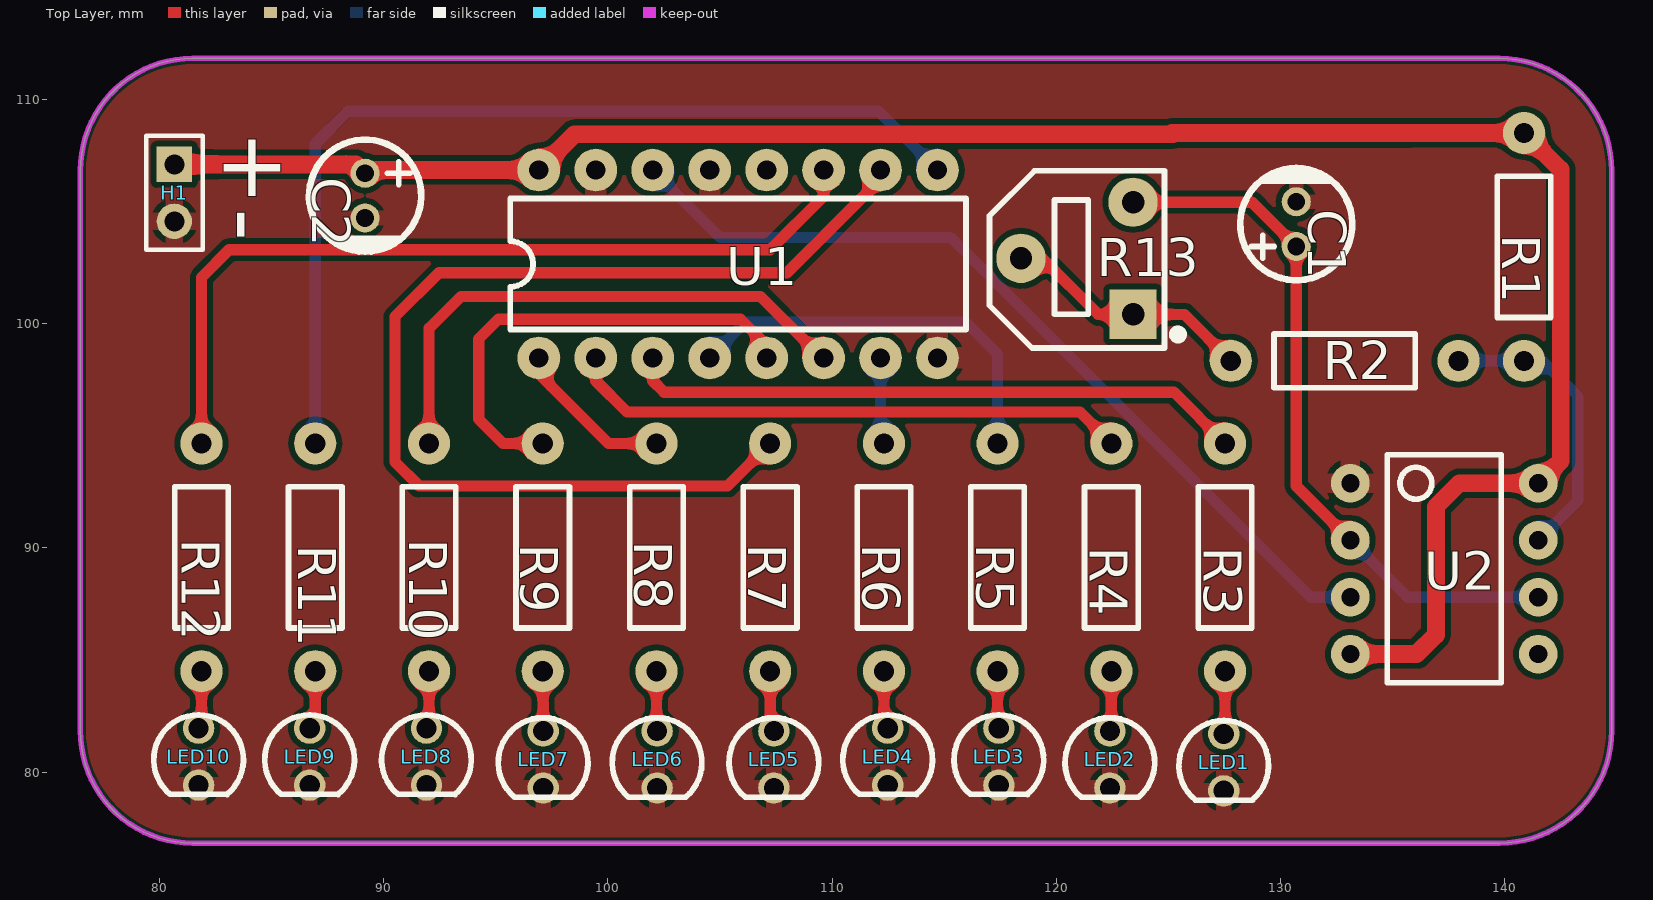
[diagram p0: Top Layer view]
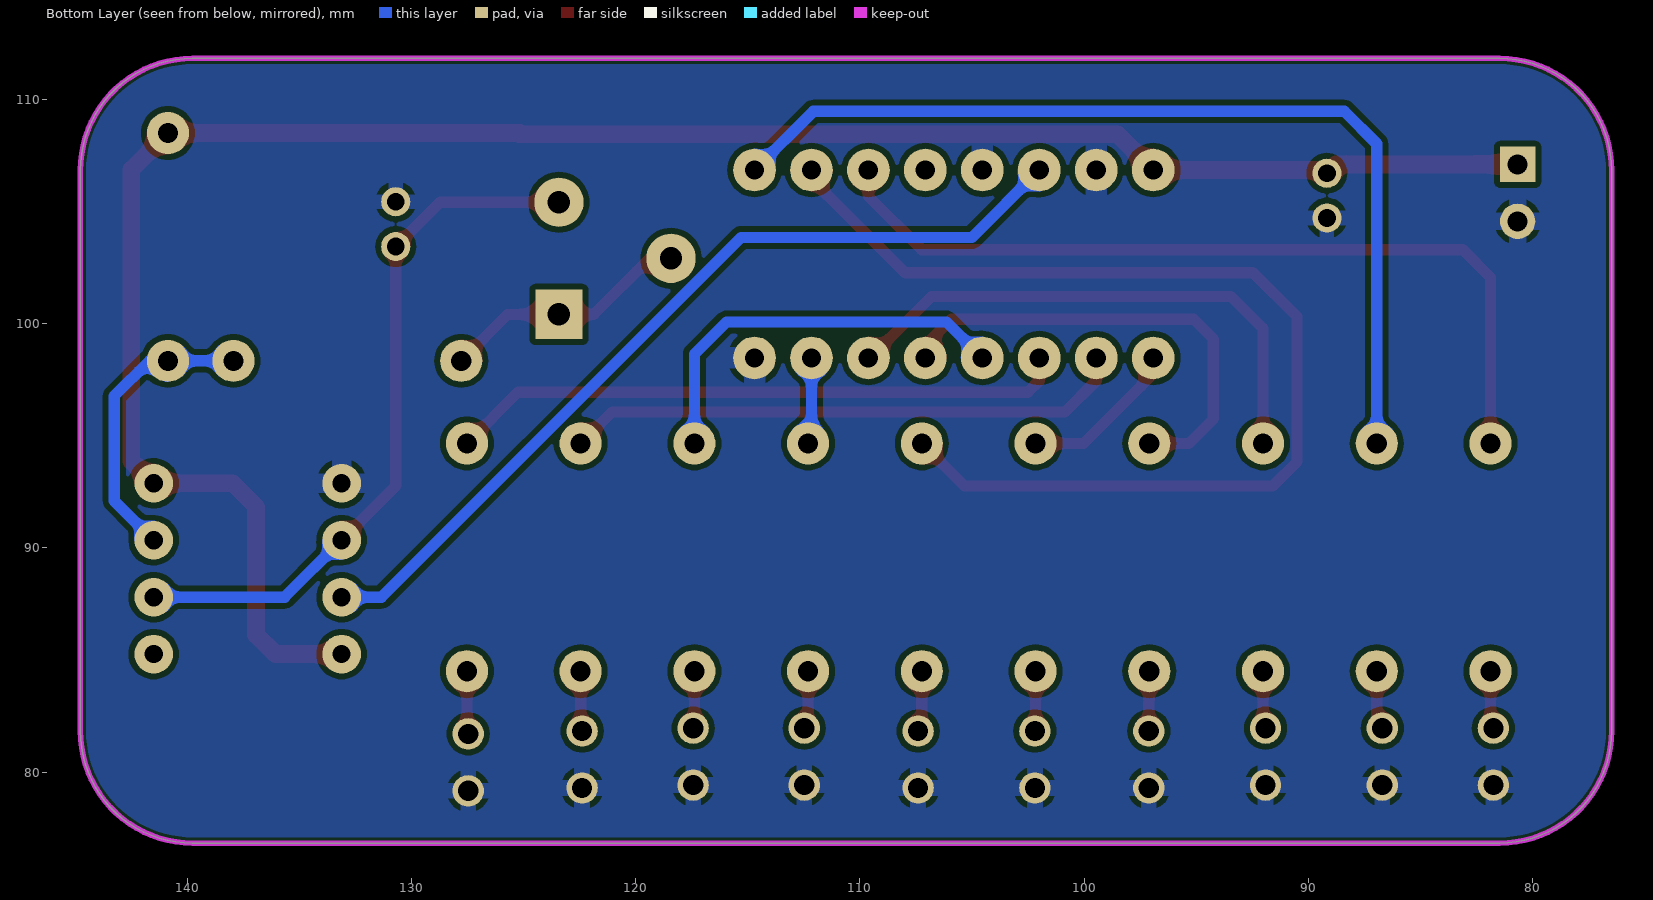
[diagram p1: Bottom Layer view, seen from below]
# Altium PCB MISC49871.pcbdoc
Units mm, origin at the board's own origin, x right, y up, seen from the top; angles counter-clockwise.
Board outline 68.29 x 35 mm, 2 copper layers (Top Layer, Bottom Layer), stack 1.58 mm thick; 28 components, 26 nets, 77 pads, 0 vias.

## Layer stack, top to bottom
Top Solder Mask Layer: solder mask 0.01, Dk 3.3
Top Layer: signal copper 0.035
Dielectric1: surface 1.51, FR4, Dk 4.5
Bottom Layer: signal copper 0.035
Bottom Solder Mask Layer: solder mask 0.01, Dk 3.3

## Board outline
76.47,106.835 cw(c81.47,106.835) 81.47,111.835 139.764,111.835 cw(c139.764,106.835) 144.764,106.835 144.764,81.835 cw(c139.764,81.835) 139.764,76.835 81.47,76.835 cw(c81.47,81.835) 76.47,81.835

## Design rules (kind name [scope] priority, off if disabled: settings)
BoardOutlineClearance GND_1 [All] p2: genericclearance=0.152 ignorepadtopadclearanceinfootprint=FALSE except(0: Text-CutoutEdge Arc-SplitContinuation Track-SplitContinuation SMDPad-SplitContinuation THPad-SplitContinuation Via-SplitContinuation Fill-SplitContinuation Region-SplitContinuation Poly-SplitContinuation Text-SplitContinuation Hole-SplitContinuation; 0.152: Arc-OutlineEdge Track-OutlineEdge SMDPad-OutlineEdge THPad-OutlineEdge Via-OutlineEdge Fill-OutlineEdge Region-OutlineEdge Text-OutlineEdge Hole-OutlineEdge Arc-CutoutEdge Track-CutoutEdge SMDPad-CutoutEdge THPad-CutoutEdge Via-CutoutEdge Fill-CutoutEdge Region-CutoutEdge Hole-CutoutEdge; 0.254: Poly-OutlineEdge Poly-CutoutEdge)
BoardOutlineClearance VCC_1 [All] p4: genericclearance=0.152 ignorepadtopadclearanceinfootprint=FALSE except(0: Text-CutoutEdge Arc-SplitContinuation Track-SplitContinuation SMDPad-SplitContinuation THPad-SplitContinuation Via-SplitContinuation Fill-SplitContinuation Region-SplitContinuation Poly-SplitContinuation Text-SplitContinuation Hole-SplitContinuation; 0.152: Arc-OutlineEdge Track-OutlineEdge SMDPad-OutlineEdge THPad-OutlineEdge Via-OutlineEdge Fill-OutlineEdge Region-OutlineEdge Text-OutlineEdge Hole-OutlineEdge Arc-CutoutEdge Track-CutoutEdge SMDPad-CutoutEdge THPad-CutoutEdge Via-CutoutEdge Fill-CutoutEdge Region-CutoutEdge Hole-CutoutEdge; 0.254: Poly-OutlineEdge Poly-CutoutEdge)
BoardOutlineClearance Plane_Default_1 [All] p6 off: genericclearance=0.152 ignorepadtopadclearanceinfootprint=FALSE except(0: Text-CutoutEdge Arc-SplitContinuation Track-SplitContinuation SMDPad-SplitContinuation THPad-SplitContinuation Via-SplitContinuation Fill-SplitContinuation Region-SplitContinuation Poly-SplitContinuation Text-SplitContinuation Hole-SplitContinuation; 0.152: Arc-OutlineEdge Track-OutlineEdge SMDPad-OutlineEdge THPad-OutlineEdge Via-OutlineEdge Fill-OutlineEdge Region-OutlineEdge Poly-OutlineEdge Text-OutlineEdge Hole-OutlineEdge Arc-CutoutEdge Track-CutoutEdge SMDPad-CutoutEdge THPad-CutoutEdge Via-CutoutEdge Fill-CutoutEdge Region-CutoutEdge Poly-CutoutEdge Hole-CutoutEdge)
BoardOutlineClearance Plane_GND_1 [All] p8 off: genericclearance=0.152 ignorepadtopadclearanceinfootprint=FALSE except(0: Text-CutoutEdge Arc-SplitContinuation Track-SplitContinuation SMDPad-SplitContinuation THPad-SplitContinuation Via-SplitContinuation Fill-SplitContinuation Region-SplitContinuation Poly-SplitContinuation Text-SplitContinuation Hole-SplitContinuation; 0.152: Arc-OutlineEdge Track-OutlineEdge SMDPad-OutlineEdge THPad-OutlineEdge Via-OutlineEdge Fill-OutlineEdge Region-OutlineEdge Poly-OutlineEdge Text-OutlineEdge Hole-OutlineEdge Arc-CutoutEdge Track-CutoutEdge SMDPad-CutoutEdge THPad-CutoutEdge Via-CutoutEdge Fill-CutoutEdge Region-CutoutEdge Poly-CutoutEdge Hole-CutoutEdge)
BoardOutlineClearance Plane_VCC_1 [All] p10 off: genericclearance=0.152 ignorepadtopadclearanceinfootprint=FALSE except(0: Text-CutoutEdge Arc-SplitContinuation Track-SplitContinuation SMDPad-SplitContinuation THPad-SplitContinuation Via-SplitContinuation Fill-SplitContinuation Region-SplitContinuation Poly-SplitContinuation Text-SplitContinuation Hole-SplitContinuation; 0.152: Arc-OutlineEdge Track-OutlineEdge SMDPad-OutlineEdge THPad-OutlineEdge Via-OutlineEdge Fill-OutlineEdge Region-OutlineEdge Poly-OutlineEdge Text-OutlineEdge Hole-OutlineEdge Arc-CutoutEdge Track-CutoutEdge SMDPad-CutoutEdge THPad-CutoutEdge Via-CutoutEdge Fill-CutoutEdge Region-CutoutEdge Poly-CutoutEdge Hole-CutoutEdge)
BoardOutlineClearance Copper_gge7237_1 [All] p12 off: genericclearance=0.152 ignorepadtopadclearanceinfootprint=FALSE except(0: Text-CutoutEdge Arc-SplitContinuation Track-SplitContinuation SMDPad-SplitContinuation THPad-SplitContinuation Via-SplitContinuation Fill-SplitContinuation Region-SplitContinuation Poly-SplitContinuation Text-SplitContinuation Hole-SplitContinuation; 0.152: Arc-OutlineEdge Track-OutlineEdge SMDPad-OutlineEdge THPad-OutlineEdge Via-OutlineEdge Fill-OutlineEdge Region-OutlineEdge Text-OutlineEdge Hole-OutlineEdge Arc-CutoutEdge Track-CutoutEdge SMDPad-CutoutEdge THPad-CutoutEdge Via-CutoutEdge Fill-CutoutEdge Region-CutoutEdge Hole-CutoutEdge; 0.254: Poly-OutlineEdge Poly-CutoutEdge)
BoardOutlineClearance Copper_gge7231_1 [All] p14 off: genericclearance=0.152 ignorepadtopadclearanceinfootprint=FALSE except(0: Text-CutoutEdge Arc-SplitContinuation Track-SplitContinuation SMDPad-SplitContinuation THPad-SplitContinuation Via-SplitContinuation Fill-SplitContinuation Region-SplitContinuation Poly-SplitContinuation Text-SplitContinuation Hole-SplitContinuation; 0.152: Arc-OutlineEdge Track-OutlineEdge SMDPad-OutlineEdge THPad-OutlineEdge Via-OutlineEdge Fill-OutlineEdge Region-OutlineEdge Text-OutlineEdge Hole-OutlineEdge Arc-CutoutEdge Track-CutoutEdge SMDPad-CutoutEdge THPad-CutoutEdge Via-CutoutEdge Fill-CutoutEdge Region-CutoutEdge Hole-CutoutEdge; 0.254: Poly-OutlineEdge Poly-CutoutEdge)
BoardOutlineClearance Default_1 [All] p16: genericclearance=0.152 ignorepadtopadclearanceinfootprint=FALSE except(0: Text-CutoutEdge Arc-SplitContinuation Track-SplitContinuation SMDPad-SplitContinuation THPad-SplitContinuation Via-SplitContinuation Fill-SplitContinuation Region-SplitContinuation Poly-SplitContinuation Text-SplitContinuation Hole-SplitContinuation; 0.152: Arc-OutlineEdge Track-OutlineEdge SMDPad-OutlineEdge THPad-OutlineEdge Via-OutlineEdge Fill-OutlineEdge Region-OutlineEdge Text-OutlineEdge Hole-OutlineEdge Arc-CutoutEdge Track-CutoutEdge SMDPad-CutoutEdge THPad-CutoutEdge Via-CutoutEdge Fill-CutoutEdge Region-CutoutEdge Hole-CutoutEdge; 0.254: Poly-OutlineEdge Poly-CutoutEdge)
Clearance GND [(InNet('GND'))] p1: gap=0.152 ignorepadtopadclearanceinfootprint=FALSE except(0: Text-Text; 0.254: Poly-Track Poly-SMDPad Poly-THPad Poly-Via Poly-Fill Poly-Region Poly-Poly Poly-Arc Poly-Text Poly-Hole)
Clearance VCC [(InNet('VCC'))] p3: gap=0.152 ignorepadtopadclearanceinfootprint=FALSE except(0: Text-Text; 0.254: Poly-Track Poly-SMDPad Poly-THPad Poly-Via Poly-Fill Poly-Region Poly-Poly Poly-Arc Poly-Text Poly-Hole)
Clearance Plane_Default [All] p5 off: gap=0.152 ignorepadtopadclearanceinfootprint=FALSE except(0: Text-Text)
Clearance Plane_GND [All] p7 off: gap=0.152 ignorepadtopadclearanceinfootprint=FALSE except(0: Text-Text)
Clearance Plane_VCC [All] p9 off: gap=0.152 ignorepadtopadclearanceinfootprint=FALSE except(0: Text-Text)
Clearance Copper_gge7237 [All] p11 off: gap=0.152 ignorepadtopadclearanceinfootprint=FALSE except(0: Text-Text; 0.254: Poly-Track Poly-SMDPad Poly-THPad Poly-Via Poly-Fill Poly-Region Poly-Poly Poly-Arc Poly-Text Poly-Hole)
Clearance Copper_gge7231 [All] p13 off: gap=0.152 ignorepadtopadclearanceinfootprint=FALSE except(0: Text-Text; 0.254: Poly-Track Poly-SMDPad Poly-THPad Poly-Via Poly-Fill Poly-Region Poly-Poly Poly-Arc Poly-Text Poly-Hole)
Clearance Default [All] p15: gap=0.152 ignorepadtopadclearanceinfootprint=FALSE except(0: Text-Text; 0.254: Poly-Track Poly-SMDPad Poly-THPad Poly-Via Poly-Fill Poly-Region Poly-Poly Poly-Arc Poly-Text Poly-Hole)
DiffPairsRouting differentialPair [All] p1: maxlimit=0.152 minlimit=0.152 mostfreqgap=0.152 toplayer_minwidth=0.127 toplayer_prefwidth=0.254 toplayer_maxwidth=2.54 toplayer_mingap=0.152 toplayer_prefgap=0.152 toplayer_maxgap=0.152 bottomlayer_minwidth=0.127 bottomlayer_prefwidth=0.254 bottomlayer_maxwidth=2.54 bottomlayer_mingap=0.152 bottomlayer_prefgap=0.152 bottomlayer_maxgap=0.152 maxuncoupledlength=0.254
HoleToHoleClearance otherClearance [All] p1: gap=0.3 allowstackedmicrovias=TRUE
Length netLength [All] p1: minlimit=0 maxlimit=0
PasteMaskExpansion Common [All] p1: expansion=0
PlaneConnect GND_4 [All] p1 off: planeconnectstyle=Relief reliefexpansion=0.508 reliefentries=4 reliefconductorwidth=0 reliefairgap=0.254
PlaneConnect VCC_4 [All] p2 off: planeconnectstyle=Relief reliefexpansion=0.508 reliefentries=4 reliefconductorwidth=0 reliefairgap=0.254
PlaneConnect Default_4 [All] p3: planeconnectstyle=Relief reliefexpansion=0.508 reliefentries=4 reliefconductorwidth=0 reliefairgap=0.254
PolygonConnect gge7231 [All] p1 off: connectstyle=Relief reliefconductorwidth=0 reliefentries=4 polygonreliefangle="90 Angle" airgapwidth=0.254 via.connectstyle=Relief via.reliefconductorwidth=0.254 via.reliefentries=4 via.polygonreliefangle="90 Angle" via.airgapwidth=0.254
PolygonConnect gge7237 [All] p2: connectstyle=Relief reliefconductorwidth=0 reliefentries=4 polygonreliefangle="90 Angle" airgapwidth=0.254 via.connectstyle=Relief via.reliefconductorwidth=0.254 via.reliefentries=4 via.polygonreliefangle="90 Angle" via.airgapwidth=0.254
RoutingVias GND_3 [(InNet('GND'))] p1: holewidth=0.305 width=0.61 viastyle="Through Hole" minholewidth=0.305 minwidth=0.61 maxholewidth=59.995 maxwidth=100.025
RoutingVias VCC_3 [(InNet('VCC'))] p2: holewidth=0.305 width=0.61 viastyle="Through Hole" minholewidth=0.305 minwidth=0.61 maxholewidth=59.995 maxwidth=100.025
RoutingVias Default_3 [All] p3: holewidth=0.305 width=0.61 viastyle="Through Hole" minholewidth=0.305 minwidth=0.61 maxholewidth=59.995 maxwidth=100.025
SolderMaskExpansion Common_1 [All] p1: expansion=0 istentingtop=FALSE
Width GND_2 [(InNet('GND'))] p1: maxlimit=25.4 minlimit=1.001 preferedwidth=1.001
Width VCC_2 [(InNet('VCC'))] p2: maxlimit=25.4 minlimit=0.8 preferedwidth=0.8
Width Default_2 [All] p3: maxlimit=25.4 minlimit=0.5 preferedwidth=0.5

## Components (designator, comment, footprint, x,y, rotation, side; value= is the part's Value field where it differs from the comment)
C1 "1uF" CAP-TH_BD5.0-P2.00-D0.8-FD 130.699,104.441 r90 top
C2 "1uF" CAP-TH_BD5.0-P2.00-D0.8-FD 89.17,105.711 r270 top
H1 "HDR-F-2.54_1x2" HDR-F-2.54_1X2 80.661,105.838 r270 top
LED1 "LED-TH-3mm_R" LED-TH_BD3.0_RED 127.466,80.438 r0 top
LED2 "LED-TH-3mm_R" LED-TH_BD3.0_RED 122.386,80.565 r0 top
LED3 "LED-TH-3mm_R" LED-TH_BD3.0_RED 117.433,80.692 r0 top
LED4 "LED-TH-3mm_R" LED-TH_BD3.0_RED 112.48,80.692 r0 top
LED5 "LED-TH-3mm_R" LED-TH_BD3.0_RED 107.4,80.565 r0 top
LED6 "LED-TH-3mm_R" LED-TH_BD3.0_RED 102.193,80.565 r0 top
LED7 "LED-TH-3mm_R" LED-TH_BD3.0_RED 97.113,80.565 r0 top
LED8 "LED-TH-3mm_R" LED-TH_BD3.0_RED 91.906,80.692 r0 top
LED9 "LED-TH-3mm_R" LED-TH_BD3.0_RED 86.699,80.692 r0 top
LED10 "LED-TH-3mm_R" LED-TH_BD3.0_RED 81.746,80.692 r0 top
R1 "2.2k" R_AXIAL-0.4 140.859,103.425 r90 top
R2 "10k" R_AXIAL-0.4 132.858,98.345 r0 top
R3 "1k" R_AXIAL-0.4 127.524,89.582 r270 top
R4 "1k" R_AXIAL-0.4 122.452,89.582 r270 top
R5 "1k" R_AXIAL-0.4 117.379,89.582 r270 top
R6 "1k" R_AXIAL-0.4 112.307,89.582 r270 top
R7 "1k" R_AXIAL-0.4 107.235,89.582 r270 top
R8 "1k" R_AXIAL-0.4 102.162,89.582 r270 top
R9 "1k" R_AXIAL-0.4 97.09,89.582 r270 top
R10 "1k" R_AXIAL-0.4 92.017,89.582 r270 top
R11 "1k" R_AXIAL-0.4 86.945,89.582 r270 top
R12 "1k" R_AXIAL-0.4 81.873,89.582 r270 top
R13 "50K" RES-ADJ-SMD_RM065-V1 120.92,102.917 r90 top
U1 "CD4017" CD4017 105.807,102.79 r0 top
U2 "NE555" DIP08-KIT 137.303,89.074 r270 top

## Footprints (in the part's own frame and the unit in brackets; to place one, negate y for a bottom-side part, rotate by r counter-clockwise, add the part's x,y. Pads: shape width x height; smd on the part's side, far side on the other; paste and mask are expansions set on the pad)
CAP-TH_BD5.0-P2.00-D0.8-FD [mm]
  round 1.3 hole 0.8: 1(-1,0) 2(1,0)
  silkscreen extent -2.5,-2.5 2.5,2.5
CD4017 [mil]
  round 75 hole 34: 1(-350,-170) 2(-250,-170) 3(-150,-170) 4(-50,-170) 5(50,-170) 6(150,-170) 7(250,-170) 8(350,-170) 9(350,160) 10(250,160) 11(150,160) 12(50,160) 13(-50,160) 14(-150,160) 15(-250,160) 16(-350,160)
  silkscreen extent -400,-120 400,110
DIP08-KIT [mil]
  round 68 hole 32: 1(-150,-165) 2(-50,-165) 3(50,-165) 4(150,-165) 5(150,165) 6(50,165) 7(-50,165) 8(-150,165)
  silkscreen extent -200,-100 200,100
HDR-F-2.54_1X2 [mil]
  rect 62x62 hole 35: 1(-50,0)
  round 62 hole 35: 2(50,0)
  silkscreen extent -100,-49 100,50
LED-TH_BD3.0_RED [mm]
  round 1.4 hole 0.9: 1(0,1.27) 2(0,-1.27)
  silkscreen extent -2,-1.69 2,1.87
R_AXIAL-0.4 [mil]
  round 74 hole 35.4: 1(-200,0) 2(200,0)
  silkscreen extent -124,-47 124,47
RES-ADJ-SMD_RM065-V1 [mm]
  rect 2.2x2.1 hole 1 paste+0 mask+0.05: 1(-2.5,-2.5)
  round 2.2 hole 1 paste+0 mask+0.05: 2(0,2.5) 3(2.5,-2.5)
  silkscreen extent -4,-4.7 3.9,3.9

## Nets (pads, with @x,y where several pads share a name; then routed paths per layer and width w, separated by ;. In a path a pad name is that pad's centre, name@x,y a point inside that pad or via, vN(x,y) a via of type N, cw(c..) or ccw(c..) an arc to the next point about the centre after c; other vN are vias at no path point)
GND: C1.2 C2.2 H1.2 LED1.2 LED2.2 LED3.2 LED4.2 LED5.2 LED6.2 LED7.2 LED8.2 LED9.2 LED10.2 U1.8 U1.13 U1.15 U2.1
LED1_1: LED1.1 R3.2 | length 2.8
  Top Layer w0.5: LED1.1@127.466,81.708 127.524,81.766 R3.2
LED2_1: LED2.1 R4.2 | length 2.7
  Top Layer w0.5: LED2.1@122.386,81.835 122.452,81.901 R4.2
LED3_1: LED3.1 R5.2 | length 2.6
  Top Layer w0.5: R5.2 117.379,82.015 LED3.1@117.433,81.962
LED4_1: LED4.1 R6.2 | length 2.6
  Top Layer w0.5: R6.2 112.307,82.135 LED4.1@112.48,81.962
LED5_1: LED5.1 R7.2 | length 2.7
  Top Layer w0.5: R7.2 107.235,82 LED5.1@107.4,81.835
LED6_1: LED6.1 R8.2 | length 2.7
  Top Layer w0.5: R8.2 102.162,81.865 LED6.1@102.193,81.835
LED7_1: LED7.1 R9.2 | length 2.7
  Top Layer w0.5: R9.2 LED7.1@97.113,81.835
LED8_1: LED8.1 R10.2 | length 2.6
  Top Layer w0.5: LED8.1@91.906,81.962 92.017,82.074 R10.2
LED9_1: LED9.1 R11.2 | length 2.6
  Top Layer w0.5: LED9.1@86.699,81.962 86.945,82.208 R11.2
LED10_1: LED10.1 R12.2 | length 2.6
  Top Layer w0.5: LED10.1@81.746,81.962 81.873,82.089 R12.2
R2_1: R2.1 R13.1 R13.2 | length 11.2
  Top Layer w0.5: R13.2@118.42,102.917 119.369,102.917 121.869,100.417 ; 121.869,100.416 R13.1 125.707,100.416 R2.1
U1_1: R8.1 U1.1 | length 7.2
  Top Layer w0.5: U1.1 96.917,97.765 100.02,94.662 R8.1
U1_2: R4.1 U1.2 | length 25.2
  Top Layer w0.5: U1.2 99.457,97.456 100.854,96.059 121.055,96.059 R4.1
U1_3: R3.1 U1.3 | length 27.7
  Top Layer w0.5: U1.3 101.997,97.456 102.505,96.948 125.238,96.948 R3.1
U1_4: R5.1 U1.4 | length 18.1
  Bottom Layer w0.5: U1.4 106.141,100.076 115.951,100.076 117.379,98.648 R5.1
U1_5: R9.1 U1.5 | length 21.1
  Top Layer w0.5: R9.1 95.329,94.663 94.234,95.758 94.234,99.314 95.123,100.203 105.918,100.203 107.076,99.045 U1.5
U1_6: R10.1 U1.6 | length 24.5
  Top Layer w0.5: R10.1 92.017,99.794 93.442,101.219 106.807,101.219 109.553,98.473 U1.6
U1_7: R6.1 U1.7 | length 3.9
  Bottom Layer w0.5: U1.7 112.157,94.812 R6.1
U1_9: R11.1 U1.9 | length 42.8
  Bottom Layer w0.5: R11.1 86.945,108.027 88.391,109.473 112.078,109.473 U1.9
U1_10: R7.1 U1.10 | length 49
  Top Layer w0.5: R7.1 105.33,92.757 91.583,92.757 90.509,93.831 90.509,100.319 92.464,102.274 107.989,102.274 112.157,106.442 U1.10
U1_11: R12.1 U1.11 | length 37.8
  Top Layer w0.5: R12.1 81.873,102.066 83.105,103.298 107.235,103.298 109.617,105.68 U1.11
U1_14: U1.14 U2.3 | length 39
  Bottom Layer w0.5: U1.14 105.004,103.847 115.291,103.847 131.334,87.804 U2.3
U2_6: C1.1 R13.3 U2.2 U2.6 | length 31.6
  Top Layer w0.5: R13.3 128.723,105.417 C1.1 130.699,92.757 U2.2
  Bottom Layer w0.5: U2.2 135.652,87.804 U2.6
U2_7: R1.1 R2.2 U2.7 | length 13.1
  Bottom Layer w0.5: R2.2 R1.1 141.685,98.345 143.256,96.774 143.256,92.106 U2.7
VCC: C2.1 H1.1 R1.2 U1.16 U2.4 U2.8 | length 93.7
  Top Layer w0.8: H1.1 88.773,107.109 C2.1 ; C2.1 89.313,106.854 U1.16 98.515,108.452 125.21,108.452 125.157,108.505 135.819,108.505 ; U2.4 136.064,85.264 136.922,86.122 136.922,91.837 137.969,92.884 U2.8 142.494,93.884 142.494,106.87 R1.2 135.819,108.505 ; 134.889,108.506 135.819,108.505
pads on no net: U1.12 U2.5

## Polygon pours and split planes (outlines as drawn)
GND on Bottom Layer (solid, remove dead copper, pour order 4): 76.327,112.395 145.034,112.395 145.288,112.141 145.288,76.962 76.581,76.962 76.327,76.708 76.327,112.014
GND on Top Layer (solid, remove dead copper, pour order 0): 76.454,112.522 144.907,112.522 145.288,112.141 145.288,76.2 76.708,76.2 76.327,76.581 76.327,112.395 76.2,112.522

## Keep-outs
Board Outline Layer:
  the board outline again, w0.254

## Other copper
Top Layer:
  drawing of 53 lines, arcs and shapes, not listed
Bottom Layer:
  region net U2_7: 139.218,98.095 139.218,98.595 139.171,98.596 139.128,98.601 139.101,98.605 139.076,98.611 139.051,98.618 139.028,98.625 139.006,98.634 138.985,98.644 138.965,98.655 138.936,98.673 138.908,98.692 138.882,98.714 138.848,98.745 138.799,98.797 138.668,98.944 138.606,99.007 138.56,99.05 138.56,97.64 138.617,97.693 138.687,97.767 138.815,97.911 138.856,97.953 138.89,97.983 138.917,98.004 138.945,98.024 138.965,98.035 138.985,98.046 139.006,98.056 139.028,98.065 139.051,98.073 139.076,98.079 139.101,98.085 139.128,98.089 139.171,98.094
  region net U1_4: 117.629,95.941 117.129,95.941 117.128,95.895 117.124,95.852 117.119,95.825 117.114,95.8 117.107,95.775 117.099,95.752 117.09,95.73 117.08,95.709 117.07,95.688 117.052,95.66 117.032,95.632 117.01,95.606 116.979,95.572 116.927,95.523 116.78,95.392 116.717,95.33 116.674,95.284 118.084,95.284 118.031,95.341 117.958,95.411 117.813,95.539 117.771,95.58 117.741,95.614 117.72,95.641 117.701,95.669 117.689,95.689 117.678,95.709 117.668,95.73 117.66,95.752 117.652,95.775 117.645,95.8 117.64,95.825 117.635,95.852 117.631,95.895
  region net U1_7: 112.407,95.941 111.907,95.941 111.905,95.898 111.9,95.854 111.892,95.81 111.881,95.766 111.867,95.722 111.842,95.656 111.812,95.591 111.778,95.528 111.74,95.466 111.687,95.389 111.631,95.317 111.602,95.284 113.012,95.284 112.98,95.317 112.922,95.37 112.678,95.57 112.581,95.656 112.537,95.7 112.498,95.744 112.464,95.789 112.45,95.811 112.437,95.833 112.427,95.855 112.418,95.877 112.412,95.898 112.408,95.92
  region net U1_9: 87.195,95.941 86.695,95.941 86.694,95.895 86.689,95.852 86.685,95.825 86.679,95.8 86.673,95.775 86.665,95.752 86.656,95.73 86.646,95.709 86.635,95.688 86.617,95.66 86.598,95.632 86.576,95.606 86.545,95.572 86.493,95.523 86.346,95.392 86.283,95.33 86.24,95.284 87.65,95.284 87.597,95.341 87.523,95.411 87.379,95.539 87.337,95.58 87.307,95.614 87.286,95.641 87.266,95.669 87.255,95.689 87.244,95.709 87.234,95.73 87.225,95.752 87.217,95.775 87.211,95.8 87.205,95.825 87.201,95.852 87.196,95.895
  region net U1_4: 105.631,99.212 105.277,99.566 105.243,99.533 105.209,99.505 105.186,99.489 105.164,99.475 105.141,99.462 105.119,99.451 105.097,99.442 105.075,99.434 105.052,99.427 105.03,99.422 104.996,99.415 104.962,99.412 104.916,99.409 104.856,99.41 104.66,99.423 104.557,99.425 104.477,99.423 105.488,98.412 105.49,98.492 105.488,98.595 105.475,98.791 105.474,98.851 105.477,98.897 105.48,98.931 105.487,98.965 105.492,98.987 105.499,99.01 105.507,99.032 105.516,99.054 105.527,99.076 105.54,99.099 105.554,99.121 105.57,99.143 105.598,99.178
  region net U1_7: 111.907,97.175 112.407,97.175 112.409,97.223 112.413,97.267 112.417,97.294 112.423,97.32 112.43,97.345 112.438,97.368 112.447,97.39 112.457,97.412 112.468,97.432 112.48,97.452 112.5,97.48 112.521,97.507 112.552,97.542 112.595,97.583 112.742,97.713 112.817,97.784 112.871,97.842 111.443,97.842 111.497,97.784 111.572,97.713 111.719,97.583 111.762,97.542 111.793,97.507 111.815,97.48 111.834,97.452 111.846,97.432 111.857,97.412 111.867,97.39 111.876,97.368 111.884,97.345 111.891,97.32 111.897,97.294 111.901,97.267 111.906,97.223
  region net U1_9: 113.957,107.948 113.603,107.594 113.636,107.56 113.664,107.525 113.68,107.503 113.694,107.481 113.707,107.458 113.718,107.436 113.727,107.414 113.735,107.392 113.742,107.369 113.748,107.347 113.754,107.313 113.758,107.279 113.76,107.233 113.759,107.173 113.746,106.977 113.744,106.874 113.746,106.794 114.757,107.805 114.677,107.807 114.574,107.805 114.378,107.792 114.318,107.791 114.272,107.794 114.238,107.797 114.204,107.804 114.182,107.809 114.16,107.816 114.137,107.824 114.115,107.833 114.093,107.844 114.071,107.857 114.048,107.871 114.026,107.887 113.991,107.915
  region net U1_14: 102.737,105.76 103.091,106.114 103.058,106.148 103.03,106.183 103.014,106.205 103,106.227 102.987,106.25 102.976,106.272 102.967,106.294 102.959,106.316 102.952,106.339 102.947,106.361 102.94,106.395 102.937,106.429 102.934,106.475 102.935,106.535 102.948,106.731 102.95,106.834 102.948,106.914 101.937,105.903 102.017,105.901 102.12,105.903 102.316,105.916 102.376,105.917 102.422,105.914 102.456,105.911 102.49,105.905 102.512,105.899 102.535,105.892 102.557,105.884 102.579,105.875 102.601,105.864 102.624,105.851 102.646,105.837 102.668,105.821 102.703,105.793
  region net U2_6: 133.767,89.336 134.12,89.689 134.092,89.719 134.068,89.749 134.047,89.778 134.035,89.798 134.024,89.818 134.015,89.838 134.006,89.858 133.996,89.888 133.988,89.918 133.982,89.948 133.977,89.979 133.974,90.022 133.972,90.087 133.977,90.29 133.975,90.384 133.974,90.398 133.058,89.482 133.14,89.479 133.335,89.483 133.413,89.483 133.456,89.481 133.497,89.476 133.528,89.471 133.558,89.463 133.589,89.454 133.608,89.446 133.628,89.437 133.648,89.427 133.668,89.415 133.687,89.402 133.717,89.38 133.747,89.355
  region net U1_14: 131.936,88.054 131.936,87.554 131.977,87.553 132.015,87.549 132.051,87.543 132.074,87.537 132.095,87.531 132.116,87.524 132.136,87.516 132.164,87.502 132.191,87.486 132.217,87.469 132.242,87.45 132.275,87.423 132.322,87.377 132.462,87.23 132.53,87.166 132.541,87.156 132.541,88.452 132.481,88.396 132.345,88.255 132.291,88.2 132.259,88.171 132.226,88.145 132.2,88.127 132.174,88.111 132.145,88.097 132.126,88.088 132.106,88.08 132.084,88.074 132.062,88.068 132.039,88.063 132.003,88.058 131.964,88.055
  region net U2_6: 140.318,88.054 140.318,87.554 140.359,87.553 140.397,87.549 140.433,87.543 140.456,87.537 140.477,87.531 140.498,87.524 140.518,87.516 140.546,87.502 140.573,87.486 140.599,87.469 140.624,87.45 140.657,87.423 140.704,87.377 140.844,87.23 140.912,87.166 140.923,87.156 140.923,88.452 140.863,88.396 140.727,88.255 140.673,88.2 140.641,88.171 140.608,88.145 140.582,88.127 140.556,88.111 140.527,88.097 140.508,88.088 140.488,88.08 140.466,88.074 140.444,88.068 140.421,88.063 140.385,88.058 140.346,88.055
  region net U2_7: 142.502,90.999 142.149,91.352 142.119,91.324 142.089,91.3 142.06,91.279 142.04,91.267 142.02,91.256 142,91.247 141.98,91.238 141.951,91.228 141.92,91.22 141.89,91.214 141.859,91.209 141.816,91.206 141.751,91.204 141.548,91.209 141.454,91.207 141.44,91.206 142.356,90.29 142.359,90.372 142.355,90.567 142.355,90.645 142.357,90.688 142.362,90.729 142.367,90.76 142.375,90.79 142.385,90.82 142.392,90.84 142.401,90.86 142.411,90.88 142.423,90.9 142.436,90.919 142.458,90.949 142.483,90.979
  region net U2_7: 139.58,98.595 139.58,98.095 139.626,98.094 139.669,98.089 139.696,98.085 139.722,98.079 139.746,98.073 139.769,98.065 139.791,98.056 139.812,98.046 139.833,98.035 139.862,98.017 139.889,97.998 139.915,97.976 139.949,97.945 139.998,97.893 140.129,97.746 140.191,97.683 140.237,97.64 140.237,99.05 140.18,98.997 140.11,98.923 139.982,98.779 139.941,98.737 139.907,98.707 139.88,98.686 139.852,98.666 139.833,98.655 139.812,98.644 139.791,98.634 139.769,98.625 139.746,98.618 139.722,98.611 139.696,98.605 139.669,98.601 139.626,98.596
  region net U2_7: 142,97.676 142.354,98.03 142.339,98.043 142.324,98.055 142.307,98.067 142.27,98.09 142.23,98.11 142.141,98.149 141.983,98.214 141.941,98.235 141.903,98.257 141.886,98.269 141.869,98.281 141.854,98.294 141.841,98.307 141.829,98.321 141.819,98.336 141.81,98.352 141.804,98.368 141.799,98.386 141.797,98.404 140.8,97.407 140.837,97.406 140.875,97.409 140.914,97.415 140.953,97.423 141.013,97.44 141.073,97.461 141.155,97.496 141.423,97.627 141.543,97.683 141.621,97.714 141.678,97.732 141.714,97.741 141.75,97.748 141.786,97.752 141.82,97.753 141.836,97.752 141.853,97.75 141.869,97.747 141.885,97.744 141.9,97.739 141.916,97.733 141.93,97.727 141.945,97.719 141.959,97.71 141.973,97.7 141.987,97.689

## Silkscreen, mask and mechanical layers (free items; w line width, h text height)
Top Silkscreen Layer:
  text "+" at 82.439,105.689 h2.95
  text "-" at 84.748,103.679 h2.95 r90